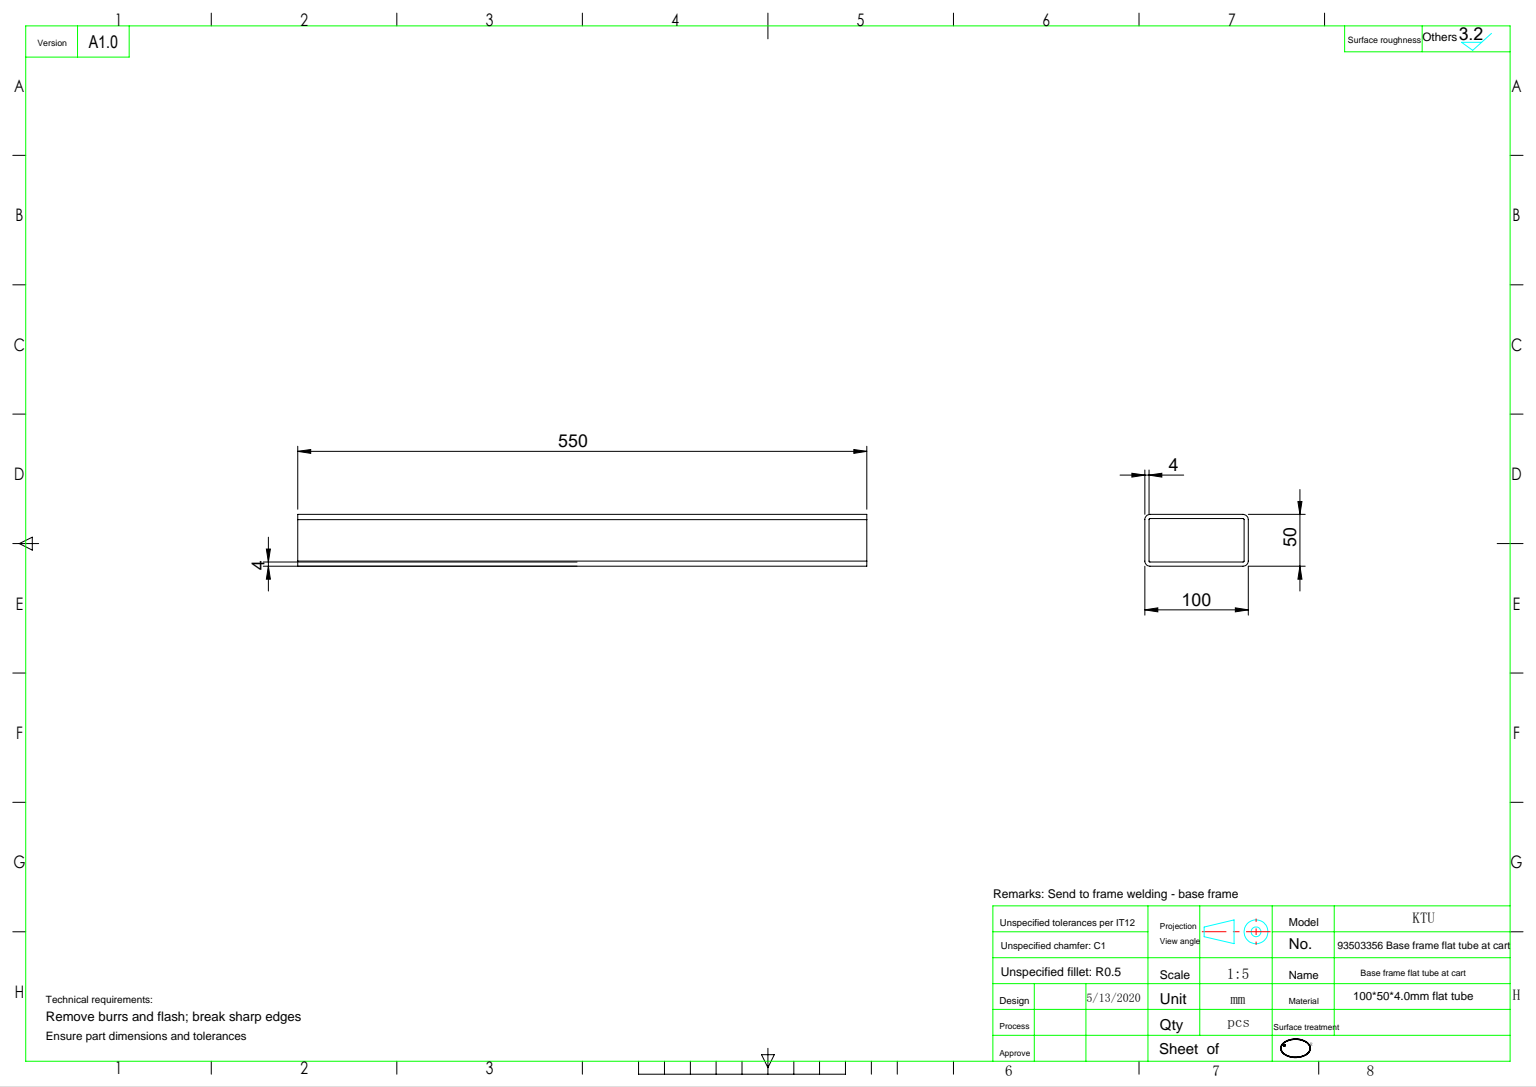
from build123d import *

# Parameters (mm, degrees)
EXTRUDE_1_DEPTH = 275


with BuildPart() as part:
    # 草图1 → 拉伸-薄壁1 (new, symmetric)
    with BuildSketch(Plane.XY):
        with BuildLine():
            Line((-45, 25), (45, 25))
            ThreePointArc((45, 25), (48.535533906, 23.535533906), (50, 20))
            Line((50, 20), (50, -20))
            ThreePointArc((50, -20), (48.535533906, -23.535533906), (45, -25))
            Line((45, -25), (-45, -25))
            ThreePointArc((-45, -25), (-48.535533906, -23.535533906), (-50, -20))
            Line((-50, -20), (-50, 20))
            ThreePointArc((-50, 20), (-48.535533906, 23.535533906), (-45, 25))
        make_face()
        with BuildLine():
            Line((-45, 21), (45, 21))
            ThreePointArc((45, 21), (45.707106781, 20.707106781), (46, 20))
            Line((46, 20), (46, -20))
            ThreePointArc((46, -20), (45.707106781, -20.707106781), (45, -21))
            Line((45, -21), (-45, -21))
            ThreePointArc((-45, -21), (-45.707106781, -20.707106781), (-46, -20))
            Line((-46, -20), (-46, 20))
            ThreePointArc((-46, 20), (-45.707106781, 20.707106781), (-45, 21))
        make_face(mode=Mode.SUBTRACT)
    extrude(amount=EXTRUDE_1_DEPTH, both=True)


solid = part.part
